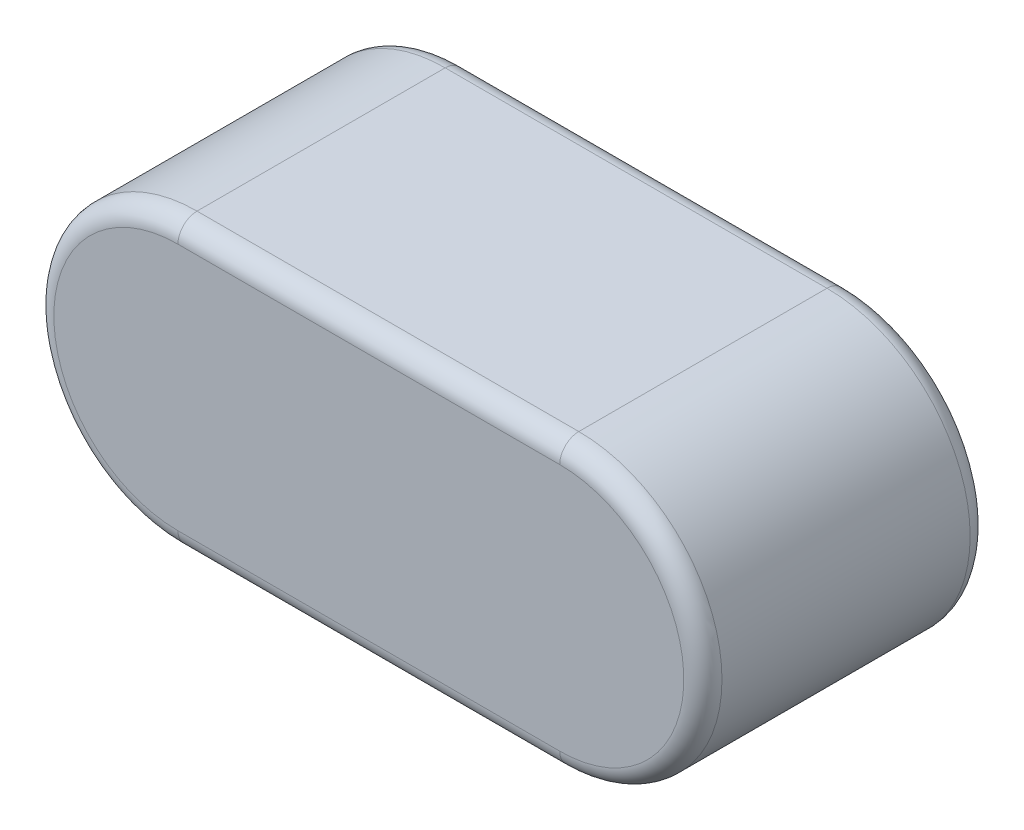
SolidWorks part; units mm, degrees
material "45"
ref_plane "基准面1" through (0, 0, 0) normal (0, 0, 1) x (1, 0, 0)
ref_plane "基准面2" through (0, 0, 0) normal (0, 1, 0) x (1, 0, 0)
ref_plane "基准面3" through (0, 0, 0) normal (1, 0, 0) x (0, 0, -1)
sketch "尺寸草图" plane through (0, 0, 0) normal (0, 0, 1) x (1, 0, 0)
  line L0 (-7, 0) -> (7, 0) construction
  point P3 (-6, 0)
  point P4 (-0.4, 0)
  point P5 (0, 0)
  point P8 (-6, 0)
  point P11 (0, 0)
sketch "草图1" plane through (0, 0, 0) normal (0, 0, 1) x (1, 0, 0)
  line L0 (-28.0599, 0) -> (30.562, 0) construction
  line L1 (-4, 3) -> (4, 3)
  line L2 (-4, -3) -> (4, -3)
  line L3 (0, 2.9108) -> (0, -2.1805) construction
  arc A0 (-4, 3) -> (-4, -3) centre (-4, 0) ccw
  arc A1 (4, 3) -> (4, -3) centre (4, 0) cw
extrude "基体-拉伸" add sketch "草图1" along normal blind 6
fillet "圆角1" radius 0.4 8 edges at (7, 0, 6) (0, 3, 6) (-7, 0, 6) (0, 3, 0) (7, 0, 0) (0, -3, 0) (-7, 0, 0) (0, -3, 6)
equation "\"D3@草图1\" = \"L@尺寸草图\""
equation "\"D1@草图1\" = \"b@尺寸草图\" / 2"
equation "\"D1@圆角1\" = \"r@尺寸草图\""
equation "\"D1@基体-拉伸\" = \"h@尺寸草图\""
